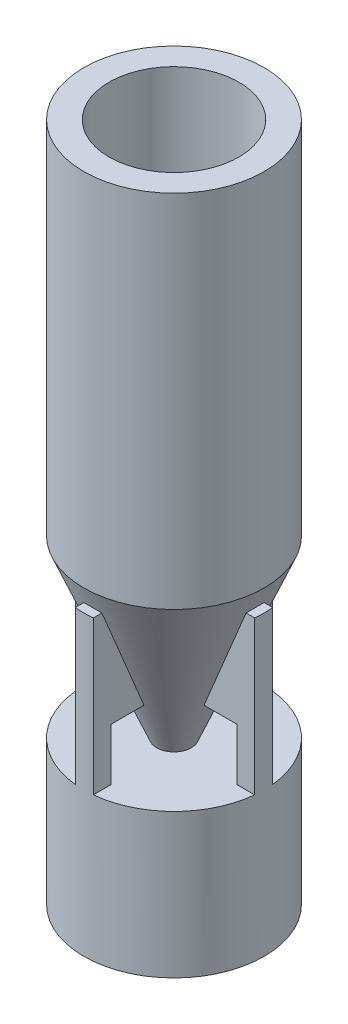
from build123d import *

# Parameters (mm, degrees)
SHELL1_T              = -70
BOSS_EXTRUDE1_DEPTH   = 25
BOSS_EXTRUDE1_2_DEPTH = 25
BOSS_EXTRUDE2_DEPTH   = 25
BOSS_EXTRUDE2_2_DEPTH = 25
SKETCH4_W             = 250
SKETCH4_H             = 400
SKETCH5_OUTSIDE_W     = 904.652
SKETCH5_OUTSIDE_H     = 904.652
SKETCH5_OUTSIDE_R     = 250
CUT_EXTRUDE1_DEPTH    = 1918.869912168


with BuildPart() as part:
    # Sketch1 → Revolve1 (revolve)
    with BuildSketch(Plane.XY, mode=Mode.PRIVATE) as revolve1_sk:
        Polygon((0, 0), (0, 1600), (250, 1600), (250, 600), align=None)
    revolve(revolve1_sk.sketch.rotate(Axis((0, 0, 0), (0, 1, 0)), 270), axis=Axis((0, 0, 0), (0, 1, 0)))

    # Shell1
    shell1_openings = [part.faces().sort_by_distance(p)[0] for p in [
        (0, 1600, 0),
    ]]
    offset(amount=SHELL1_T, openings=shell1_openings, kind=Kind.INTERSECTION)


with BuildPart() as body_2:
    # Sketch2 → Boss-Extrude1 (new, symmetric)
    with BuildSketch(Plane.XY):
        Polygon((-108.333333333, 260), (-199.333333333, 260), (-199.333333333, 0), (-250, 0), (-250, 540), (-225, 540), align=None)
    extrude(amount=BOSS_EXTRUDE1_DEPTH, both=True)


with BuildPart() as body_3:
    # Sketch2 → Boss-Extrude1 2 (new, symmetric)
    with BuildSketch(Plane.XY):
        Polygon((225, 540), (108.333333333, 260), (199.333333333, 260), (199.333333333, 0), (250, 0), (250, 540), align=None)
    extrude(amount=BOSS_EXTRUDE1_2_DEPTH, both=True)


with BuildPart() as body_4:
    # Sketch3 → Boss-Extrude2 (new, symmetric)
    with BuildSketch(Plane(origin=(0, 0, 0), x_dir=(0, 0, -1), z_dir=(1, 0, 0))):
        Polygon((-250, 0), (-199.333333333, 0), (-199.333333333, 260), (-108.333333333, 260), (-225, 540), (-250, 540), align=None)
    extrude(amount=BOSS_EXTRUDE2_DEPTH, both=True)


with BuildPart() as body_5:
    # Sketch3 → Boss-Extrude2 2 (new, symmetric)
    with BuildSketch(Plane(origin=(0, 0, 0), x_dir=(0, 0, -1), z_dir=(1, 0, 0))):
        Polygon((108.333333333, 260), (225, 540), (250, 540), (250, 0), (199.333333333, 0), (199.333333333, 260), align=None)
    extrude(amount=BOSS_EXTRUDE2_2_DEPTH, both=True)


    add(body_4.part)  # Revolve2 merges body 4

    add(body_3.part)  # Revolve2 merges body 3

    add(body_2.part)  # Revolve2 merges body 2
    # Sketch4 → Revolve2 (revolve)
    with BuildSketch(Plane.XY, mode=Mode.PRIVATE) as revolve2_sk:
        with Locations((125, -85)):
            Rectangle(SKETCH4_W, SKETCH4_H)
    revolve(revolve2_sk.sketch.rotate(Axis((0, 115, 0), (0, -1, 0)), 180), axis=Axis((0, 115, 0), (0, -1, 0)))

    # Sketch5 outside → Cut-Extrude1 (cut, through all)
    with BuildSketch(Plane.XZ.offset(285)):
        Rectangle(SKETCH5_OUTSIDE_W, SKETCH5_OUTSIDE_H)
        with Locations(Location((0, 0, 0), (0, 0, 180))):
            Circle(SKETCH5_OUTSIDE_R, mode=Mode.SUBTRACT)
    extrude(amount=-CUT_EXTRUDE1_DEPTH, mode=Mode.SUBTRACT)


solid = Compound([part.part, body_5.part])
